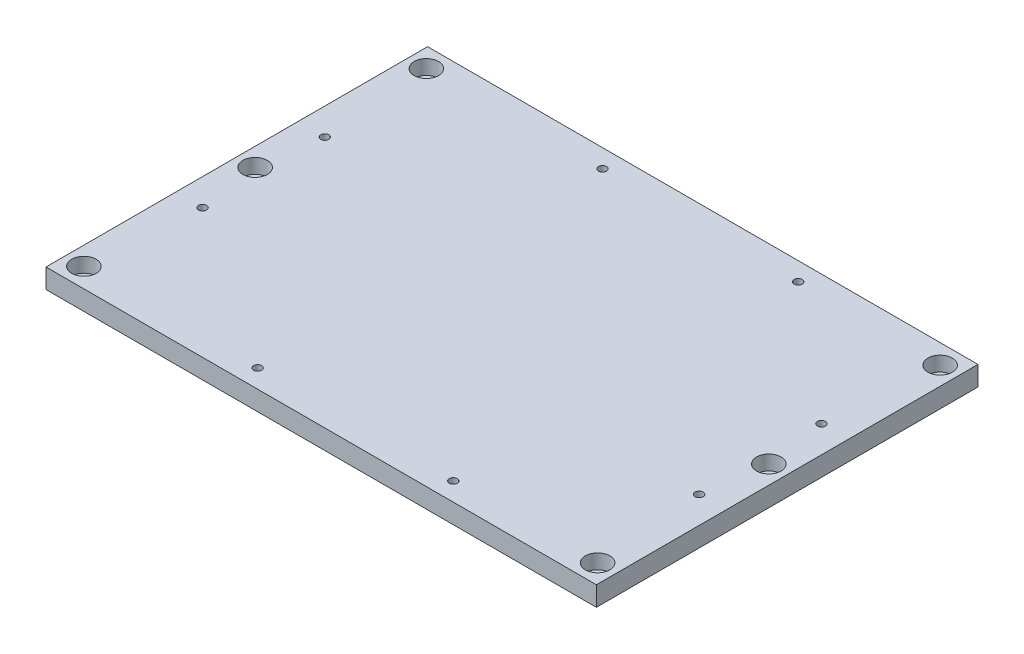
from build123d import *

# Parameters (mm, degrees)
SKETCH1_W                                         = 225
SKETCH1_H                                         = 156
EXTRUDE1_DEPTH                                    = 4
M5_SOCKET_HEAD_CAP_SCREW_COUNTERBORE1_D           = 5.5
M5_SOCKET_HEAD_CAP_SCREW_COUNTERBORE1_CBORE_D     = 10
M5_SOCKET_HEAD_CAP_SCREW_COUNTERBORE1_CBORE_DEPTH = 6
M4_TAPPED_HOLE1_D                                 = 3.3
M4_TAPPED_HOLE2_D                                 = 3.3


with BuildPart() as part:
    # Sketch1 → Extrude1 (new, symmetric)
    with BuildSketch(Plane(origin=(0, 0, 0), x_dir=(1, 0, 0), z_dir=(0, 1, 0))):
        Rectangle(SKETCH1_W, SKETCH1_H)
    extrude(amount=EXTRUDE1_DEPTH, both=True)

    # M5 Socket Head Cap Screw Counterbore1 (through all)
    with Locations(Plane(origin=(105, 4, 70), x_dir=(0, 0, 1), z_dir=(0, 1, 0))):
        with Locations((0, 0), (-70, 0), (-140, 0)):
            m5_socket_head_cap_screw_counterbore1 = CounterBoreHole(M5_SOCKET_HEAD_CAP_SCREW_COUNTERBORE1_D / 2, M5_SOCKET_HEAD_CAP_SCREW_COUNTERBORE1_CBORE_D / 2, M5_SOCKET_HEAD_CAP_SCREW_COUNTERBORE1_CBORE_DEPTH)

    # Mirror1: M5 Socket Head Cap Screw Counterbore1 across plane
    add(m5_socket_head_cap_screw_counterbore1.mirror(Plane(origin=(0, 0, 0), x_dir=(0, 0, 1), z_dir=(1, 0, 0))), mode=Mode.SUBTRACT)

    # M4 Tapped Hole1 (through all)
    with Locations(Plane(origin=(101.5, 4, 25), x_dir=(0, 0, 1), z_dir=(0, 1, 0))):
        with Locations((0, 0), (-50, 0)):
            m4_tapped_hole1 = Hole(M4_TAPPED_HOLE1_D / 2)

    # M4 Tapped Hole2 (through all)
    with Locations(Plane(origin=(-33.5, 4, 70.5), x_dir=(0, 0, 1), z_dir=(0, 1, 0))):
        with Locations((0, 0), (0, 80)):
            m4_tapped_hole2 = Hole(M4_TAPPED_HOLE2_D / 2)

    # Mirror2: M4 Tapped Hole1 across plane
    add(m4_tapped_hole1.mirror(Plane(origin=(0, 0, 0), x_dir=(0, 0, 1), z_dir=(1, 0, 0))), mode=Mode.SUBTRACT)

    # Mirror3: M4 Tapped Hole2 across plane
    add(m4_tapped_hole2.mirror(Plane.XY), mode=Mode.SUBTRACT)


solid = part.part
